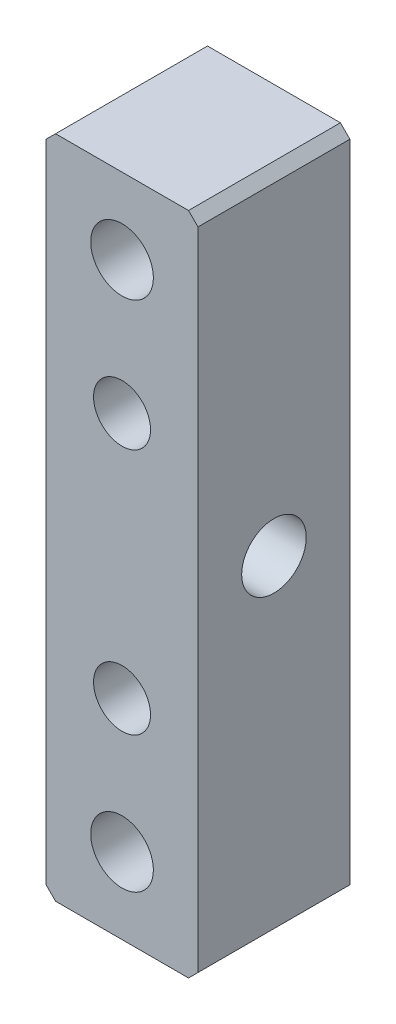
SolidWorks part; units mm, degrees
material "Q235-A"
ref_plane "Front Plane" through (0, 0, 0) normal (0, 0, 1) x (1, 0, 0)
ref_plane "Top Plane" through (0, 0, 0) normal (0, 1, 0) x (1, 0, 0)
ref_plane "Right Plane" through (0, 0, 0) normal (1, 0, 0) x (0, 0, -1)
sketch "Sketch1" plane through (0, 0, 0) normal (0, 0, 1) x (1, 0, 0)
  line L0 (0, 70) -> (0, 0)
  dimension "D2" = 70
extrude "Extrude-Thin1" add sketch "Sketch1" along normal blind 16 thin
chamfer "Chamfer1" distance 1 angle 45 4 edges at (-16, 70, 8) (0, 70, 8) (0, 0, 8) (-16, 0, 8)
hole_wizard "Size mm blind dowel hole 1" positions "Sketch2" profile "Sketch3" hole size "Ø6.0" standard "GB" end condition through all
sketch "Sketch2" plane through (0, 0, 16) normal (0, 0, 1) x (1, 0, 0)
  line L0 (-16, 69) -> (-16, 1) construction
  line L4 (-15, 70) -> (-1, 70) construction
  line L5 (-1, 0) -> (-15, 0) construction
  point P0 (-8, 48)
  point P2 (-8, 22)
  dimension "D1" = 8
  dimension "D2" = 22
  dimension "D3" = 22
sketch "Sketch3" plane through (-8, 48, 16) normal (1, 0, 0) x (0, -1, 0)
  line L0 (0, 0) -> (0, 16)
  line L1 (0, 16) -> (3, 16)
  line L2 (3, 16) -> (3, 0)
  line L5 (3, 0) -> (0, 0)
  line L11 (0, -6.35) -> (0, 107.95) construction
  dimension "通孔孔直径" = 6
  dimension "通孔孔深度" = 16
hole_wizard "M8 Tapped Hole1" positions "Sketch6" profile "Sketch5" tap size "M8" standard "GB" end condition through all
sketch "Sketch6" plane through (-16, 0, 0) normal (-1, 0, 0) x (0, 0, 1)
  line L0 (16, 69) -> (16, 1) construction
  line L7 (0, 35) -> (16, 35) construction
  line L8 (0, 69) -> (0, 1) construction
  point P4 (8, 35)
  dimension "D2" = 8
sketch "Sketch5" plane through (-16, 35, 8) normal (0, 1, 0) x (0, 0, 1)
  line L0 (0, 0) -> (0, 16)
  line L1 (0, 16) -> (3.4, 16)
  line L2 (3.4, 16) -> (3.4, 0)
  line L5 (3.4, 0) -> (0, 0)
  line L11 (0, -6.35) -> (0, 107.95) construction
  dimension "通孔螺纹孔钻头直径" = 6.8
  dimension "通孔螺纹孔钻头深度" = 16
cosmetic thread "Cosmetic thread 2" parameters "D2"=8
hole_wizard "M6 Clearance Hole1" positions "Sketch7" profile "Sketch9" hole size "M6" standard "GB" end condition through all
sketch "Sketch7" plane through (0, 0, 16) normal (0, 0, 1) x (1, 0, 0)
  line L0 (-8, 70) -> (-8, 0) construction
  line L1 (-15, 70) -> (-1, 70) construction
  line L2 (-1, 0) -> (-15, 0) construction
  line L4 (-16, 35) -> (0, 35) construction
  line L5 (-16, 69) -> (-16, 1) construction
  line L6 (0, 69) -> (0, 1) construction
  point P0 (-8, 62)
  point P2 (-8, 8)
  dimension "D1" = 8
sketch "Sketch9" plane through (-8, 62, 16) normal (1, 0, 0) x (0, -1, 0)
  line L0 (0, 0) -> (0, 16)
  line L1 (0, 16) -> (3.3, 16)
  line L2 (3.3, 16) -> (3.3, 0)
  line L5 (3.3, 0) -> (0, 0)
  line L11 (0, -6.35) -> (0, 107.95) construction
  dimension "通孔孔直径" = 6.6
  dimension "通孔孔深度" = 16
